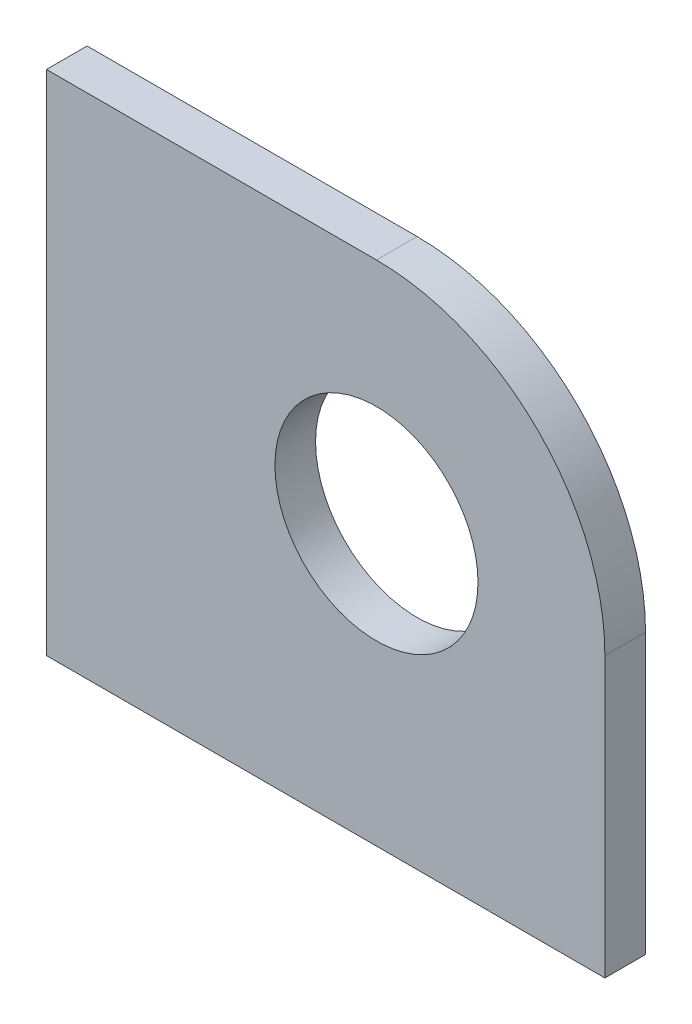
SolidWorks part; units mm, degrees
material "Q235B"
ref_plane "Front Plane" through (0, 0, 0) normal (0, 0, 1) x (1, 0, 0)
ref_plane "Top Plane" through (0, 0, 0) normal (0, 1, 0) x (1, 0, 0)
ref_plane "Right Plane" through (0, 0, 0) normal (1, 0, 0) x (0, 0, -1)
sketch "Sketch1" plane through (0, 0, 0) normal (0, 0, 1) x (1, 0, 0)
  line L1 (0, 0) -> (110, 0)
  line L2 (0, 0) -> (0, 100)
  line L3 (0, 100) -> (65, 100)
  line L4 (110, 0) -> (110, 55)
  arc A0 (65, 100) -> (110, 55) centre (65, 55) cw
  circle A1 centre (65, 55) radius 20
  dimension "D3" = 45
  dimension "D4" = 40
  dimension "D1" = 110
  dimension "D2" = 100
extrude "Boss-Extrude1" add sketch "Sketch1" along normal blind 8
